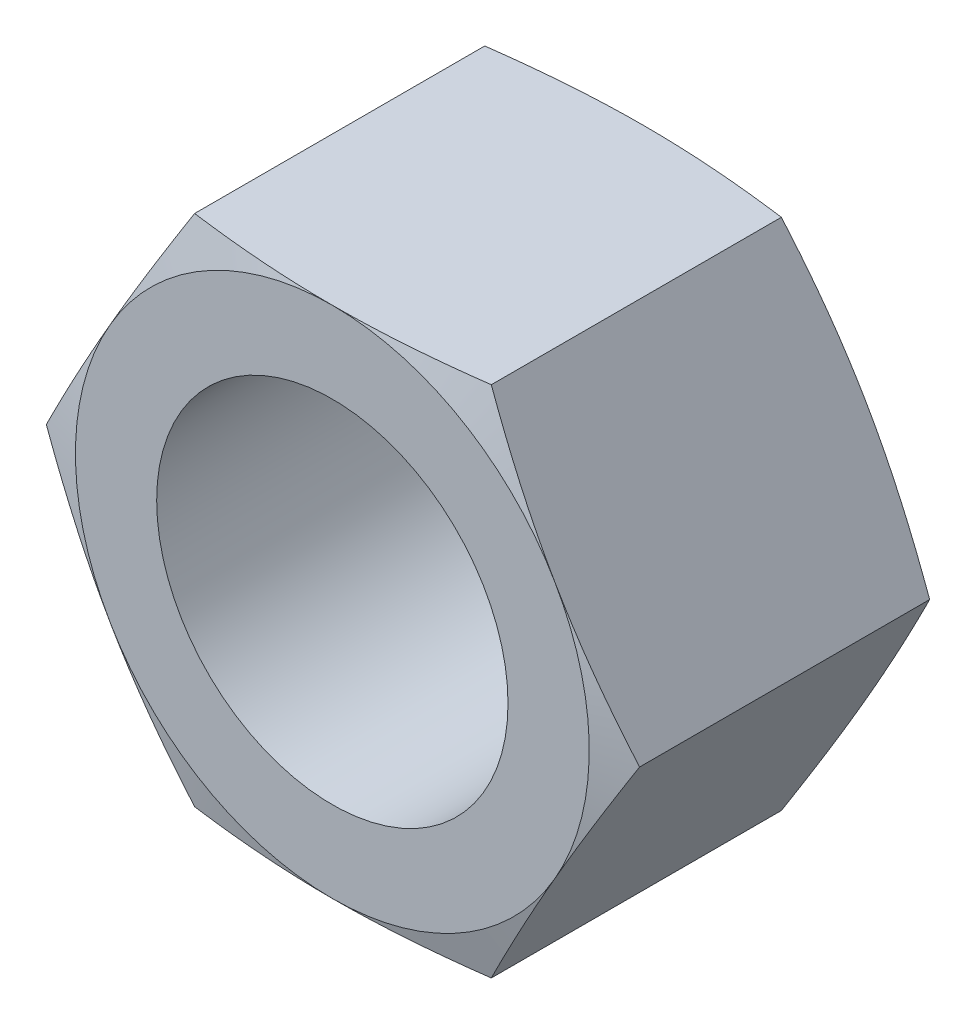
from build123d import *

# Parameters (mm, degrees)
SKETCH_1_R          = 18
EXTRUDE_519_DEPTH   = 31.9
SKETCH_2_OUTSIDE_W  = 363.728
SKETCH_2_OUTSIDE_H  = 355.584
SKETCH_2_OUTSIDE_R  = 26.322842148
CUT_EXTRUDE_1_DEPTH = 38
CUT_EXTRUDE_1_DRAFT = -75
SKETCH_3_OUTSIDE_W  = 363.728
SKETCH_3_OUTSIDE_H  = 355.584
SKETCH_3_OUTSIDE_R  = 26.322842148
CUT_EXTRUDE_2_DEPTH = 38
CUT_EXTRUDE_2_DRAFT = -75


with BuildPart() as part:
    # 草图1 → Extrude 519 (new body)
    with BuildSketch(Plane.XY):
        Polygon((15.1975, 26.322842148), (-15.1975, 26.322842148), (-30.395, 0), (-15.1975, -26.322842148), (15.1975, -26.322842148), (30.395, 0), align=None)
        Circle(SKETCH_1_R, mode=Mode.SUBTRACT)
    extrude(amount=EXTRUDE_519_DEPTH)


with BuildPart() as cut_extrude_1_tool:
    # 草图2 outside → 切除-拉伸1 (with draft: the straight prism first)
    with BuildSketch(Plane(origin=(0, 0, 0), x_dir=(-1, 0, 0), z_dir=(0, 0, -1))):
        Rectangle(SKETCH_2_OUTSIDE_W, SKETCH_2_OUTSIDE_H)
        Circle(SKETCH_2_OUTSIDE_R, mode=Mode.SUBTRACT)
    extrude(amount=-CUT_EXTRUDE_1_DEPTH)
    # 切除-拉伸1: the draft: its side faces are tilted about the plane it starts from
    cut_extrude_1_sides = [cut_extrude_1_tool.faces().sort_by_distance(p)[0] for p in [
        (0, -177.792, 19),
        (-181.864, 0, 19),
        (0, 177.792, 19),
        (181.864, 0, 19),
        (26.322842148, 0, 19),
    ]]
    draft(cut_extrude_1_sides, Plane(origin=(0, 0, 0), x_dir=(-1, 0, 0), z_dir=(0, 0, -1)), CUT_EXTRUDE_1_DRAFT)


with BuildPart() as part_1:
    add(part.part)

    # 切除-拉伸1: cut by cut_extrude_1_tool
    add(cut_extrude_1_tool.part, mode=Mode.SUBTRACT)


with BuildPart() as cut_extrude_2_tool:
    # 草图3 outside → 切除-拉伸2 (with draft: the straight prism first)
    with BuildSketch(Plane.XY.offset(31.9)):
        Rectangle(SKETCH_3_OUTSIDE_W, SKETCH_3_OUTSIDE_H)
        Circle(SKETCH_3_OUTSIDE_R, mode=Mode.SUBTRACT)
    extrude(amount=-CUT_EXTRUDE_2_DEPTH)
    # 切除-拉伸2: the draft: its side faces are tilted about the plane it starts from
    cut_extrude_2_sides = [cut_extrude_2_tool.faces().sort_by_distance(p)[0] for p in [
        (0, -177.792, 12.9),
        (181.864, 0, 12.9),
        (0, 177.792, 12.9),
        (-181.864, 0, 12.9),
        (-26.322842148, 0, 12.9),
    ]]
    draft(cut_extrude_2_sides, Plane.XY.offset(31.9), CUT_EXTRUDE_2_DRAFT)


with BuildPart() as part_2:
    add(part_1.part)

    # 切除-拉伸2: cut by cut_extrude_2_tool
    add(cut_extrude_2_tool.part, mode=Mode.SUBTRACT)


solid = part_2.part
